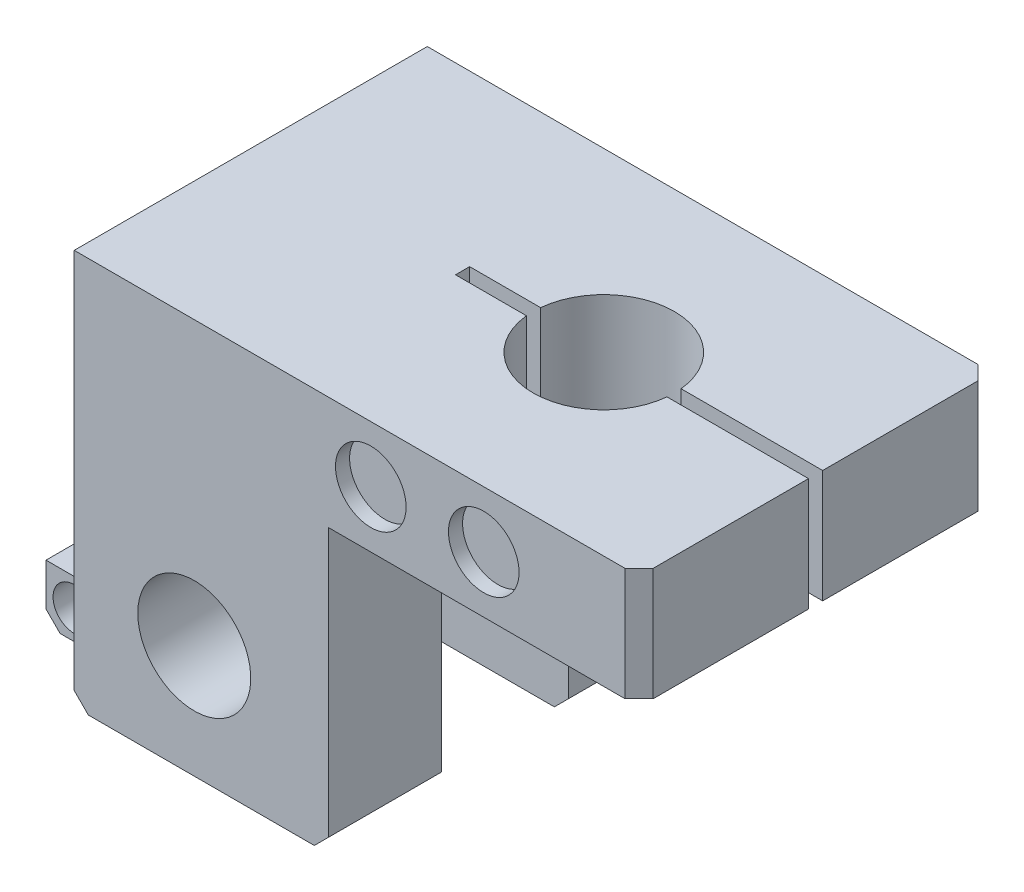
SolidWorks part; units mm, degrees
material "Q235-A"
ref_plane "Front Plane" through (0, 0, 0) normal (0, 0, 1) x (1, 0, 0)
ref_plane "Top Plane" through (0, 0, 0) normal (0, 1, 0) x (1, 0, 0)
ref_plane "Right Plane" through (0, 0, 0) normal (1, 0, 0) x (0, 0, -1)
sketch "Sketch1" plane through (0, 0, 0) normal (0, 1, 0) x (1, 0, 0)
  line L1 (0, 0) -> (40, 0)
  line L2 (0, 0) -> (0, -25)
  line L3 (0, -25) -> (40, -25)
  line L4 (40, 0) -> (40, -25)
  dimension "D1" = 40
  dimension "D2" = 25
extrude "Boss-Extrude1" add sketch "Sketch1" along normal blind 8
sketch "Sketch3" plane through (0, 8, 0) normal (0, 1, 0) x (1, 0, 0)
  line L0 (25, -12.5) -> (40, -12.5) construction
  line L1 (40, -25) -> (40, 0) construction
  circle A0 centre (25, -12.5) radius 5
  dimension "D1" = 10
  dimension "D2" = 15
extrude "Cut-Extrude1" cut sketch "Sketch3" against normal through all
sketch "Sketch4" plane through (0, 8, 0) normal (0, 1, 0) x (1, 0, 0)
  line L0 (40, -25) -> (40, 0) construction
  line L1 (15, -12) -> (40, -12)
  line L2 (15, -12) -> (15, -13)
  line L3 (15, -13) -> (40, -13)
  line L4 (40, -12) -> (40, -13)
  line L5 (15, -12.5) -> (0, -12.5) construction
  line L6 (0, 0) -> (0, -25) construction
  dimension "D1" = 1
  dimension "D2" = 25
extrude "Cut-Extrude2" cut sketch "Sketch4" against normal through all
sketch "Sketch7" plane through (0, 0, 0) normal (0, -1, 0) x (1, 0, 0)
  line L1 (0, 0) -> (18, 0)
  line L2 (0, 0) -> (0, 8)
  line L3 (0, 8) -> (18, 8)
  line L4 (18, 0) -> (18, 8)
  line L5 (0, 25) -> (18, 25)
  line L6 (0, 25) -> (0, 17)
  line L7 (0, 17) -> (18, 17)
  line L8 (18, 25) -> (18, 17)
  dimension "D1" = 8
  dimension "D2" = 8
  dimension "D3" = 18
extrude "Boss-Extrude2" add sketch "Sketch7" along normal blind 20
chamfer "Chamfer2" distance 1 angle 45 4 edges at (40, 4, 25) (40, 4, 0) (18, -20, 21) (18, -20, 4)
sketch "Sketch8" plane through (0, 0, 0) normal (0, 0, -1) x (-1, 0, 0)
  line L0 (-8.5, -12) -> (-8.5, -20) construction
  line L1 (0, -20) -> (-17, -20) construction
  circle A0 centre (-8.5, -12) radius 4
  dimension "D2" = 8
  dimension "D1" = 8
extrude "Cut-Extrude3" cut sketch "Sketch8" against normal through all
sketch "Sketch9" plane through (0, 0, 0) normal (0, 0, -1) x (-1, 0, 0)
  line L0 (-40, 0) -> (-40, 8) construction
  circle A0 centre (-29, 4) radius 2.5
  circle A1 centre (-21, 4) radius 2.5
  dimension "D1" = 8
  dimension "D2" = 11
extrude "Cut-Extrude4" cut sketch "Sketch9" against normal blind 1
sketch "Sketch10" plane through (0, 0, 25) normal (0, 0, 1) x (1, 0, 0)
  circle A1 centre (21, 4) radius 2.5
  circle A2 centre (21, 4) radius 2.5
  circle A3 centre (29, 4) radius 2.5
  circle A4 centre (29, 4) radius 2.5
  dimension "D1" = 0
  dimension "D2" = 0
extrude "Cut-Extrude5" cut sketch "Sketch10" against normal blind 1
sketch "Sketch11" plane through (0, 0, 0) normal (-1, 0, 0) x (0, 0, 1)
  line L0 (12.5, 9.1555) -> (12.5, -21.5201) construction
  line L1 (21, -20) -> (21, -16)
  line L2 (8, -20) -> (4, -20)
  line L3 (8, -20) -> (8, -16)
  line L4 (8, -16) -> (4, -16)
  line L5 (4, -20) -> (4, -16)
  line L6 (17, -16) -> (21, -16)
  line L7 (17, -20) -> (17, -16)
  line L8 (17, -20) -> (21, -20)
  dimension "D1" = 4
  dimension "D2" = 4
extrude "Boss-Extrude3" add sketch "Sketch11" along normal blind 6
sketch "Sketch12" plane through (0, 0, 4) normal (0, 0, -1) x (-1, 0, 0)
  line L0 (6, -16) -> (6, -20) construction
  circle A0 centre (4, -18) radius 1.5
  dimension "D1" = 2
extrude "Cut-Extrude6" cut sketch "Sketch12" against normal blind 20
chamfer "Chamfer4" distance 1 angle 45 4 edges at (0, -20, 23) (-6, -20, 19) (-6, -20, 6) (0, -20, 2)
